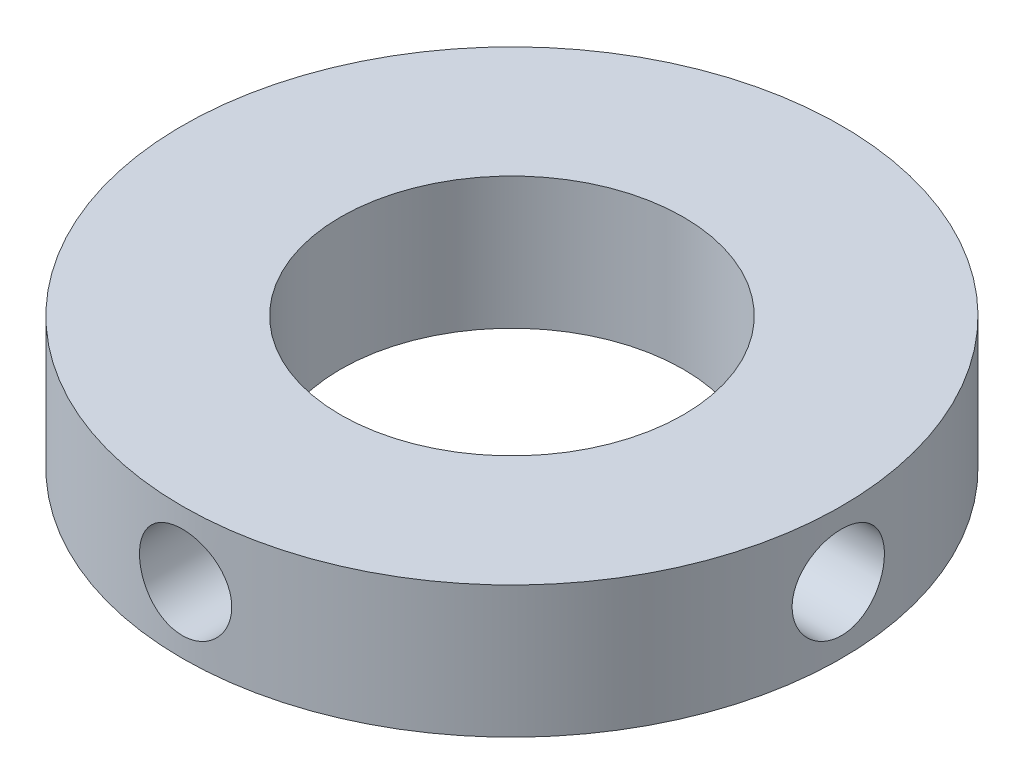
from build123d import *

# Parameters (mm, degrees)
SKETCH1_R                  = 50
BOSS_EXTRUDE1_DEPTH        = 20
M56X4_0_TAPPED_HOLE1_D     = 52
M56X4_0_TAPPED_HOLE1_DEPTH = 124
M56X4_0_TAPPED_HOLE1_TIP   = 15.622376095
CIRPATTERN1_COUNT          = 4


with BuildPart() as part:
    # Sketch1 → Boss-Extrude1 (new body)
    with BuildSketch(Plane(origin=(0, 0, 0), x_dir=(1, 0, 0), z_dir=(0, 1, 0))):
        with Locations(Location((0, 0, 0), (0, 0, 270))):
            Circle(SKETCH1_R)
    extrude(amount=BOSS_EXTRUDE1_DEPTH)

    # M56x4.0 Tapped Hole1
    with Locations(Plane(origin=(0, 20, 0), x_dir=(1, 0, 0), z_dir=(0, 1, 0))):
        with Locations((0, 0)):
            Hole(M56X4_0_TAPPED_HOLE1_D / 2, depth=M56X4_0_TAPPED_HOLE1_DEPTH)
            with Locations((0, 0, -(M56X4_0_TAPPED_HOLE1_DEPTH + M56X4_0_TAPPED_HOLE1_TIP / 2))):  # 118° drill point
                Cone(0, M56X4_0_TAPPED_HOLE1_D / 2, M56X4_0_TAPPED_HOLE1_TIP, mode=Mode.SUBTRACT)

    # Sketch5 → Ø14.0 (14) Diameter Hole1 (revolve, cut)
    with BuildSketch(Plane(origin=(0, 10, 50), x_dir=(0, -1, 0), z_dir=(1, 0, 0))):
        Polygon((0, 0), (0, 20), (7, 15.793975667), (7, 0), align=None)
    f_14_0_14_diameter_hole1 = revolve(axis=Axis((0, 10, 56.35), (0, 0, -1)), mode=Mode.SUBTRACT)

    # CirPattern1: Ø14.0 (14) Diameter Hole1 ×4 about axis
    cirpattern1_axis = Axis((0, 20, 0), (0, 1, 0))
    for i in range(1, CIRPATTERN1_COUNT):
        add(f_14_0_14_diameter_hole1.rotate(cirpattern1_axis, i * 360 / CIRPATTERN1_COUNT), mode=Mode.SUBTRACT)


solid = part.part
